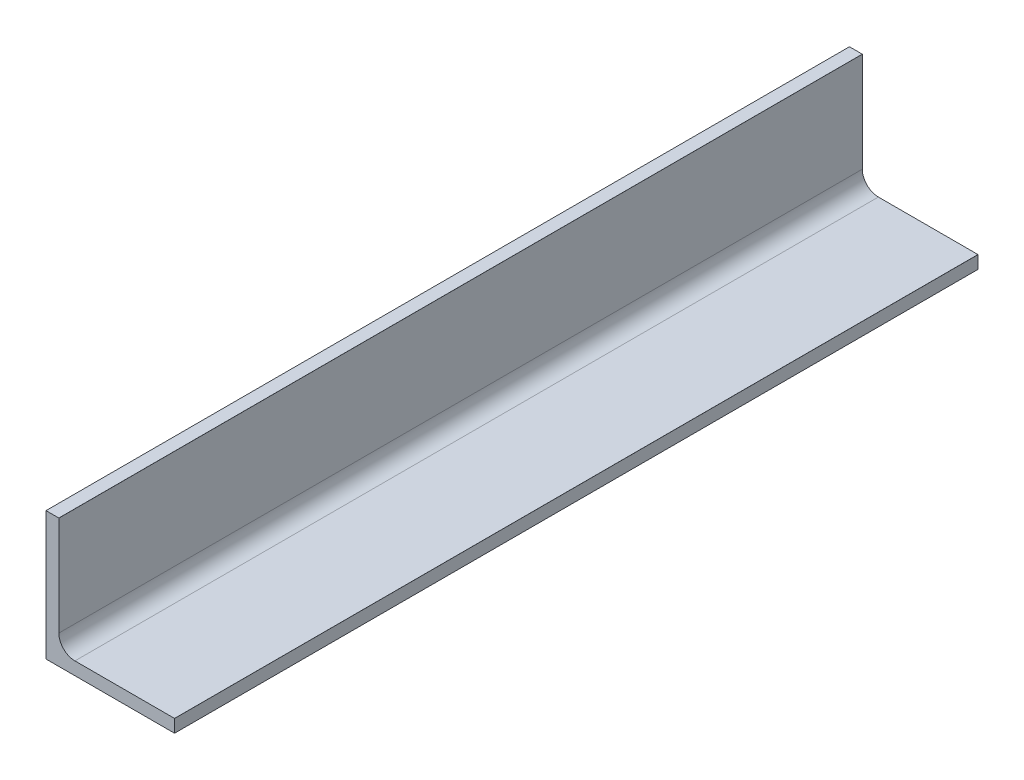
from build123d import *

# Parameters (mm, degrees)
EXTRUDE_1_DEPTH = 250


with BuildPart() as part:
    # 草图1 → 拉伸1 (new body)
    with BuildSketch(Plane.XY):
        with BuildLine():
            Line((0, 0), (0, 40))
            Line((0, 40), (3.99, 40))
            ThreePointArc((3.99, 40), (3.997071068, 39.997071068), (4, 39.99))
            Line((4, 39.99), (4, 9))
            ThreePointArc((4, 9), (5.464466094, 5.464466094), (9, 4))
            Line((9, 4), (39.99, 4))
            ThreePointArc((39.99, 4), (39.997071068, 3.997071068), (40, 3.99))
            Line((40, 3.99), (40, 0))
            Line((40, 0), (0, 0))
        make_face()
    extrude(amount=EXTRUDE_1_DEPTH)


solid = part.part
